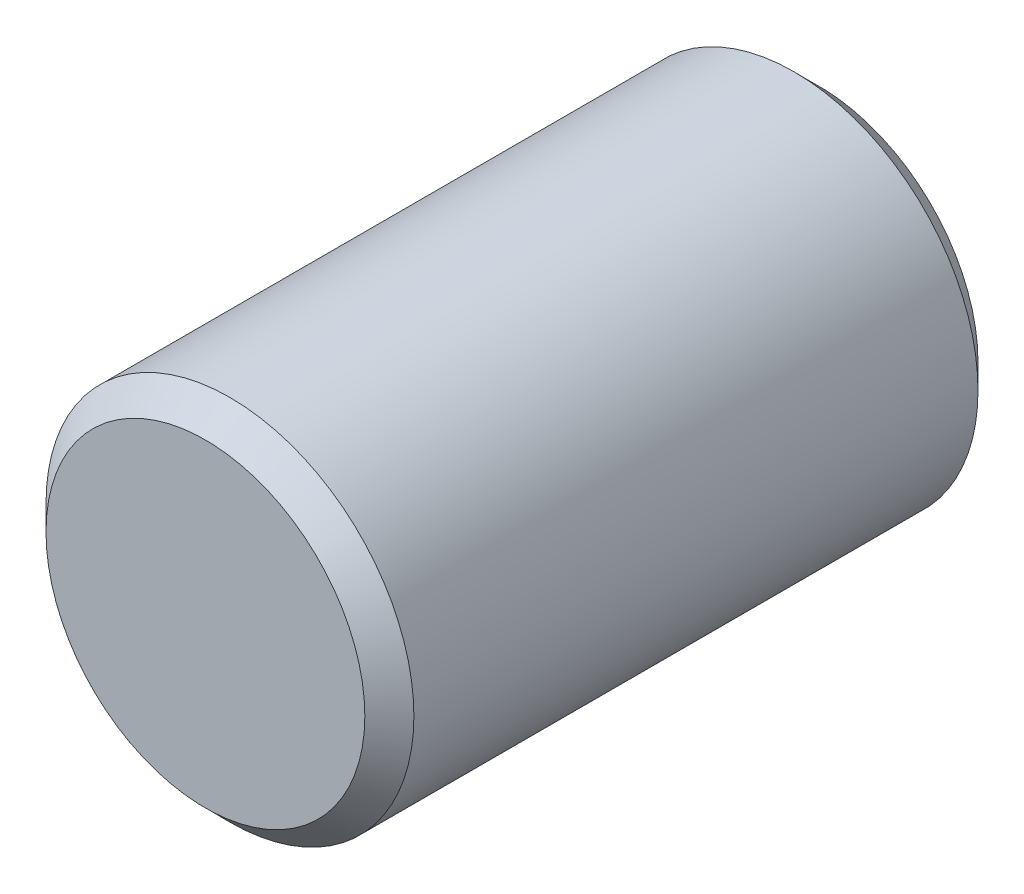
SolidWorks part; units mm, degrees
ref_plane "Front Plane" through (0, 0, 0) normal (0, 0, 1) x (1, 0, 0)
ref_plane "Top Plane" through (0, 0, 0) normal (0, 1, 0) x (1, 0, 0)
ref_plane "Right Plane" through (0, 0, 0) normal (1, 0, 0) x (0, 0, -1)
other "Configuration Table"
sketch "Sketch1" plane through (0, 0, 0) normal (0, 0, 1) x (1, 0, 0)
  circle A0 centre (0, 0) radius 1.5
  dimension "D1" = 3
extrude "Boss-Extrude1" add sketch "Sketch1" along normal blind 5
chamfer "Chamfer1" distance 0.2 angle 45 2 edges at (1.5, 0, 0) (1.5, 0, 5)
